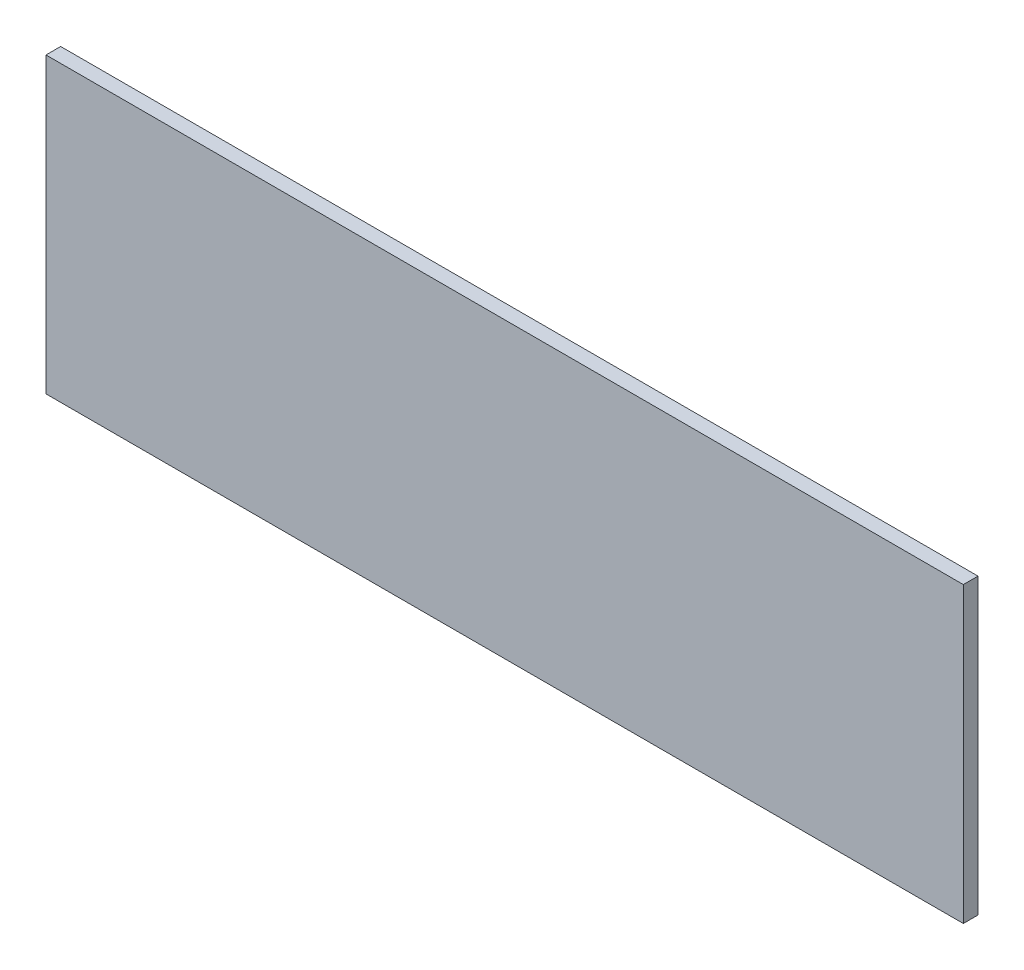
from build123d import *

# Parameters (mm, degrees)
SKETCH_1_W      = 125
SKETCH_1_H      = 40
EXTRUDE_1_DEPTH = 2


with BuildPart() as part:
    # 草图1 → 凸台-拉伸1 (new body)
    with BuildSketch(Plane.XY):
        Rectangle(SKETCH_1_W, SKETCH_1_H)
    extrude(amount=EXTRUDE_1_DEPTH)


solid = part.part
